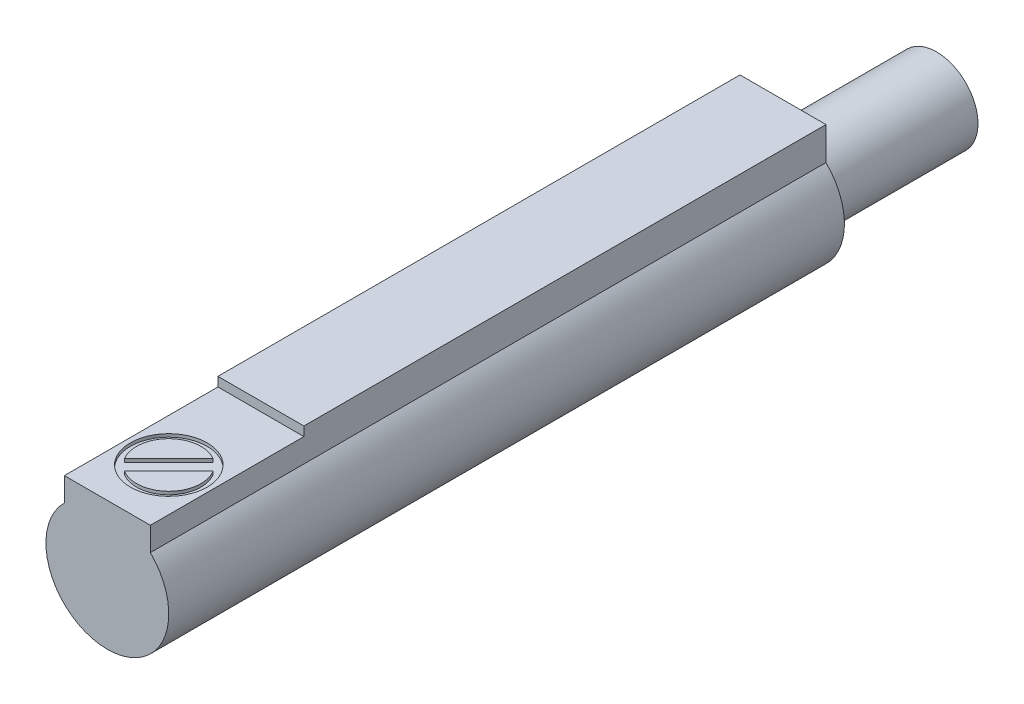
from build123d import *

# Parameters (mm, degrees)
BOSS_EXTRUDE1_DEPTH = 22
SKETCH2_W           = 2.8
SKETCH2_H           = 0.3
CUT_EXTRUDE1_DEPTH  = 5
SKETCH3_R           = 1.25
SKETCH3_R_2         = 1.05
CUT_EXTRUDE2_DEPTH  = 0.1
CUT_EXTRUDE3_DEPTH  = 0.1
SKETCH5_W           = 1.35
SKETCH5_H           = 5


with BuildPart() as part:
    # Sketch1 → Boss-Extrude1 (new body)
    with BuildSketch(Plane.XY):
        with BuildLine():
            Line((1.4, 1.428285686), (1.4, 2.5))
            Line((1.4, 2.5), (-1.4, 2.5))
            Line((-1.4, 2.5), (-1.4, 1.428285686))
            ThreePointArc((-1.4, 1.428285686), (0, -2), (1.4, 1.428285686))
        make_face()
    extrude(amount=-BOSS_EXTRUDE1_DEPTH)

    # Sketch2 → Cut-Extrude1 (cut)
    with BuildSketch(Plane.XY):
        with Locations((0, 2.35)):
            Rectangle(SKETCH2_W, SKETCH2_H)
    extrude(amount=-CUT_EXTRUDE1_DEPTH, mode=Mode.SUBTRACT)

    # Sketch3 → Cut-Extrude2 (cut)
    with BuildSketch(Plane(origin=(0, 2.2, 0), x_dir=(1, 0, 0), z_dir=(0, 1, 0))):
        with Locations(Location((0, 2, 0), (0, 0, 270))):
            Circle(SKETCH3_R)
        with Locations(Location((0, 2, 0), (0, 0, 270))):
            Circle(SKETCH3_R_2, mode=Mode.SUBTRACT)
    extrude(amount=-CUT_EXTRUDE2_DEPTH, mode=Mode.SUBTRACT)

    # Sketch4 → Cut-Extrude3 (cut)
    with BuildSketch(Plane(origin=(0, 2.2, 0), x_dir=(1, 0, 0), z_dir=(0, 1, 0))):
        with BuildLine():
            Line((-0.54433356, 1.10211305), (0.89788695, 2.54433356))
            ThreePointArc((0.89788695, 2.54433356), (0.74246212, 2.74246212), (0.54433356, 2.89788695))
            Line((0.54433356, 2.89788695), (-0.89788695, 1.45566644))
            ThreePointArc((-0.89788695, 1.45566644), (-0.74246212, 1.25753788), (-0.54433356, 1.10211305))
        make_face()
    extrude(amount=-CUT_EXTRUDE3_DEPTH, mode=Mode.SUBTRACT)

    # Sketch5 → Revolve1 (revolve)
    with BuildSketch(Plane(origin=(0, 0, 0), x_dir=(1, 0, 0), z_dir=(0, 1, 0)), mode=Mode.PRIVATE) as revolve1_sk:
        with Locations((-0.675, 24.5)):
            Rectangle(SKETCH5_W, SKETCH5_H)
    revolve(revolve1_sk.sketch.rotate(Axis((0, 0, -27), (0, 0, 1)), 180), axis=Axis((0, 0, -27), (0, 0, 1)))


solid = part.part
